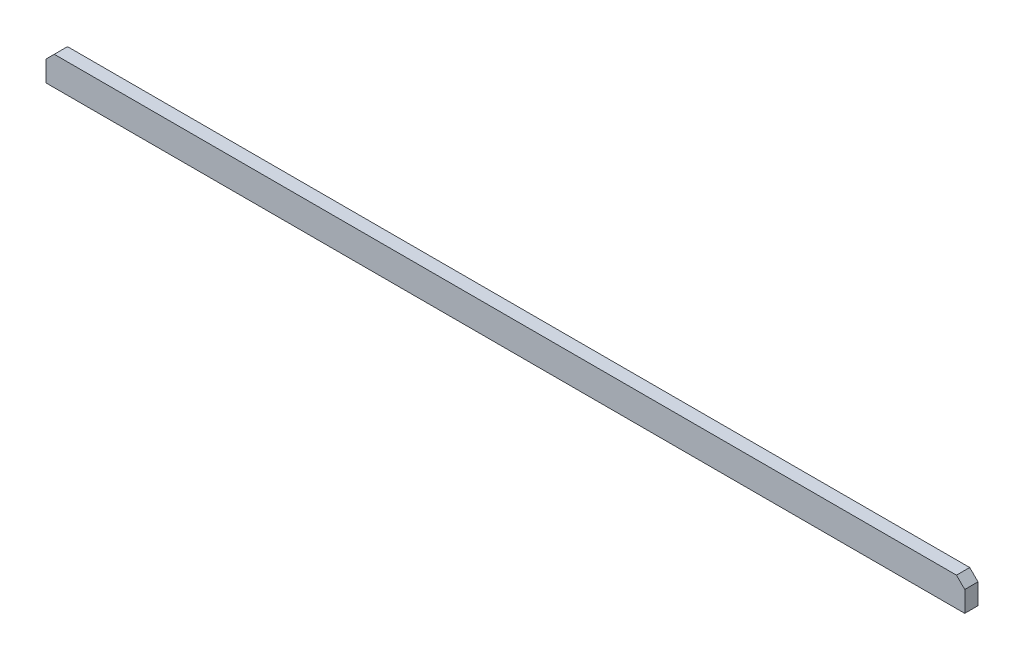
from build123d import *

# Parameters (mm, degrees)
SKETCH1_W           = 1110
SKETCH1_H           = 35
BOSS_EXTRUDE1_DEPTH = 16
CHAMFER1_SIZE       = 10


with BuildPart() as part:
    # Sketch1 → Boss-Extrude1 (new body)
    with BuildSketch(Plane.XY):
        with Locations((490.486370787, 15.12341466)):
            Rectangle(SKETCH1_W, SKETCH1_H)
    extrude(amount=BOSS_EXTRUDE1_DEPTH)

    # Chamfer1
    chamfer1_edges = [part.edges().sort_by_distance(p)[0] for p in [
        (1045.486370787, 32.62341466, 8),
        (-64.513629213, 32.62341466, 8),
    ]]
    chamfer(chamfer1_edges, length=CHAMFER1_SIZE)


solid = part.part
